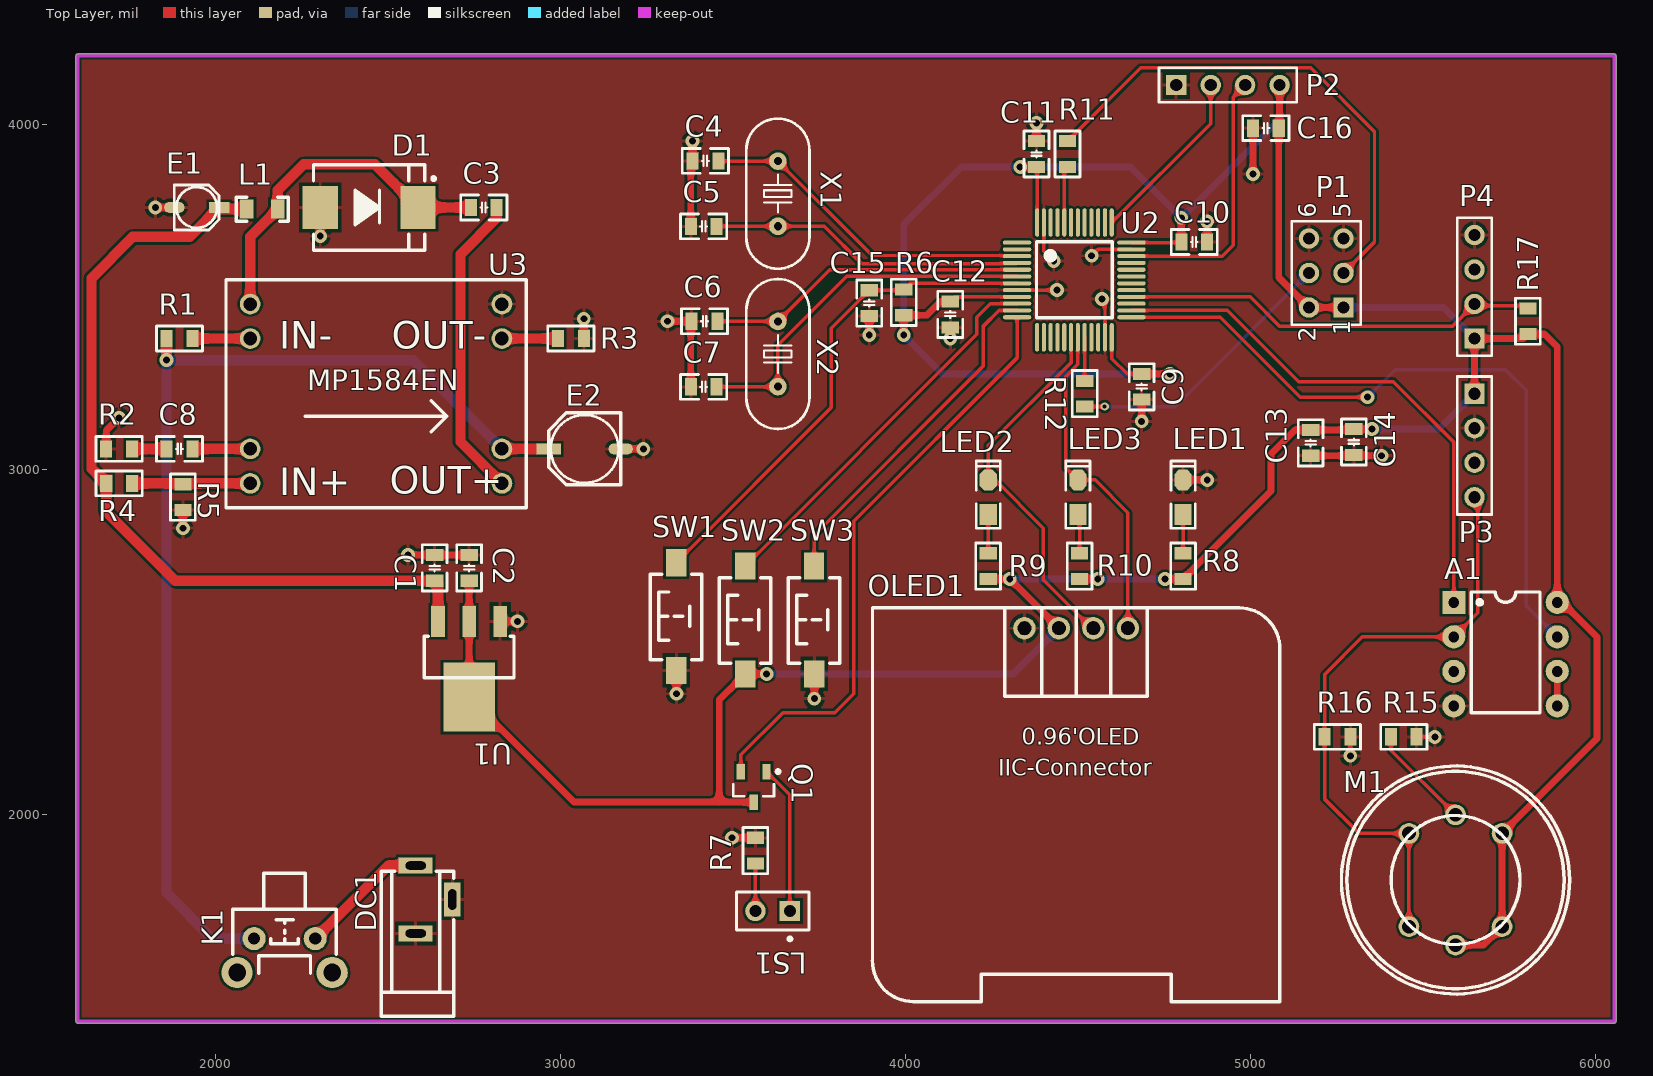
[diagram p0: Top Layer view]
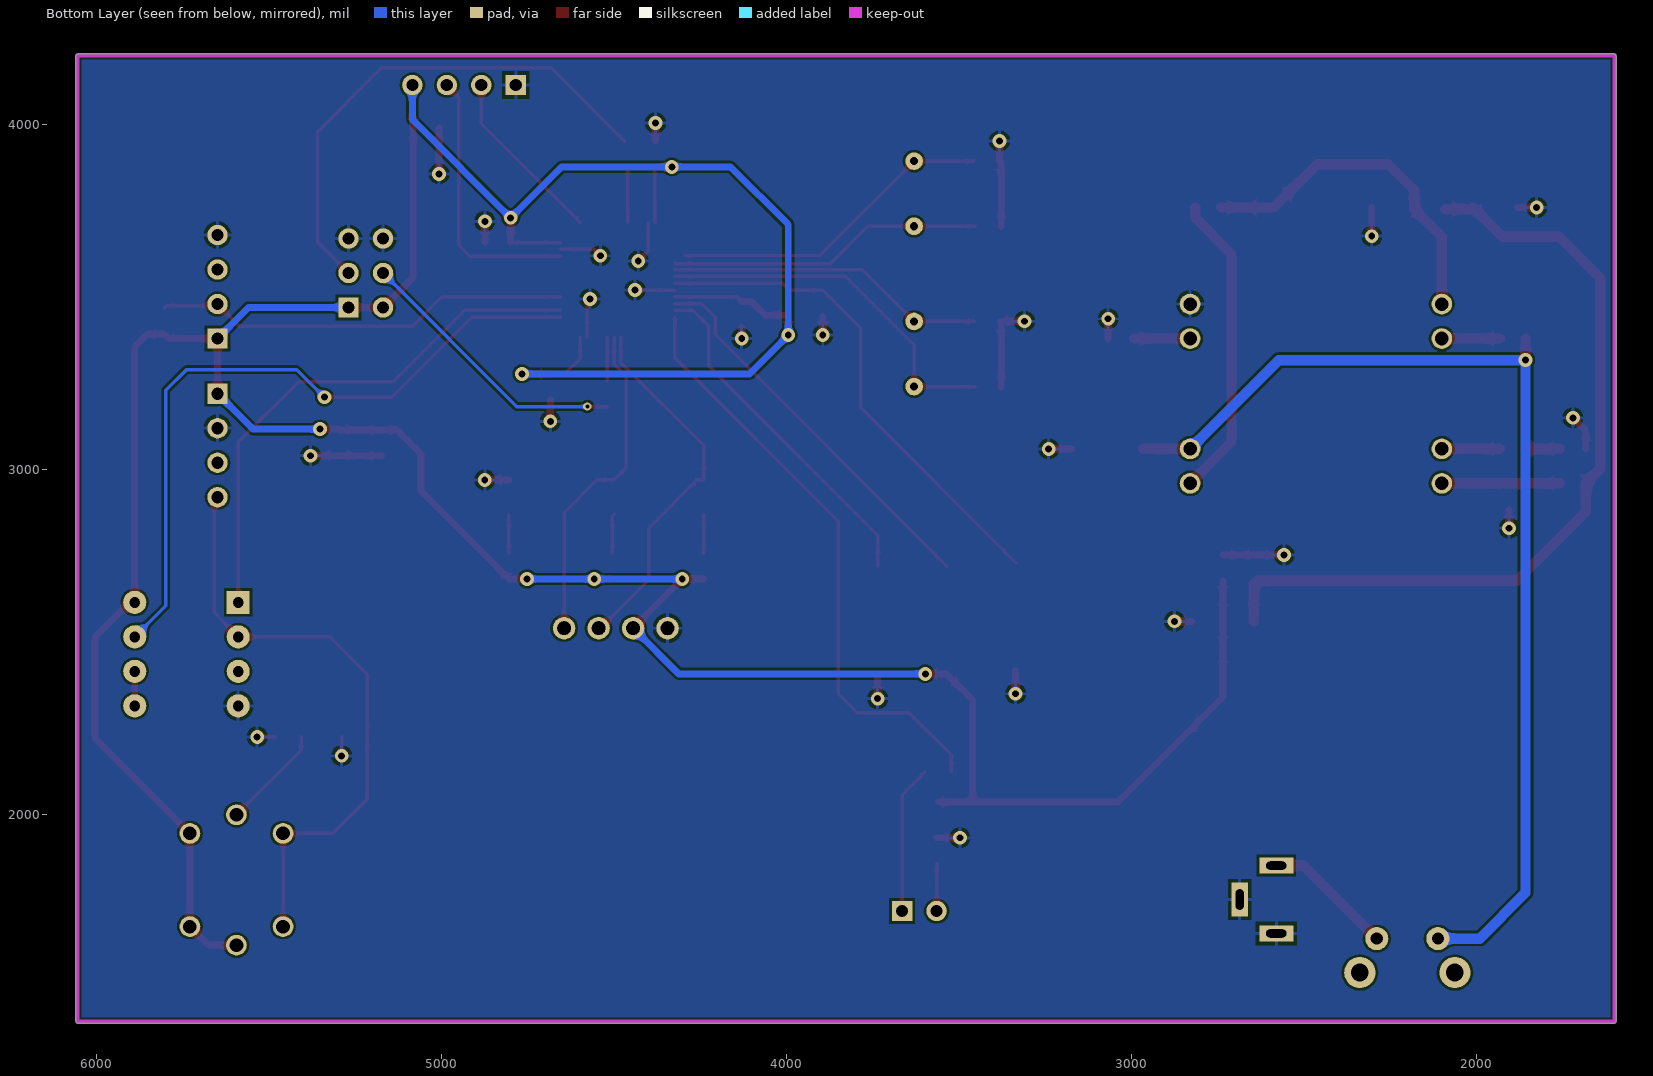
[diagram p1: Bottom Layer view, seen from below]
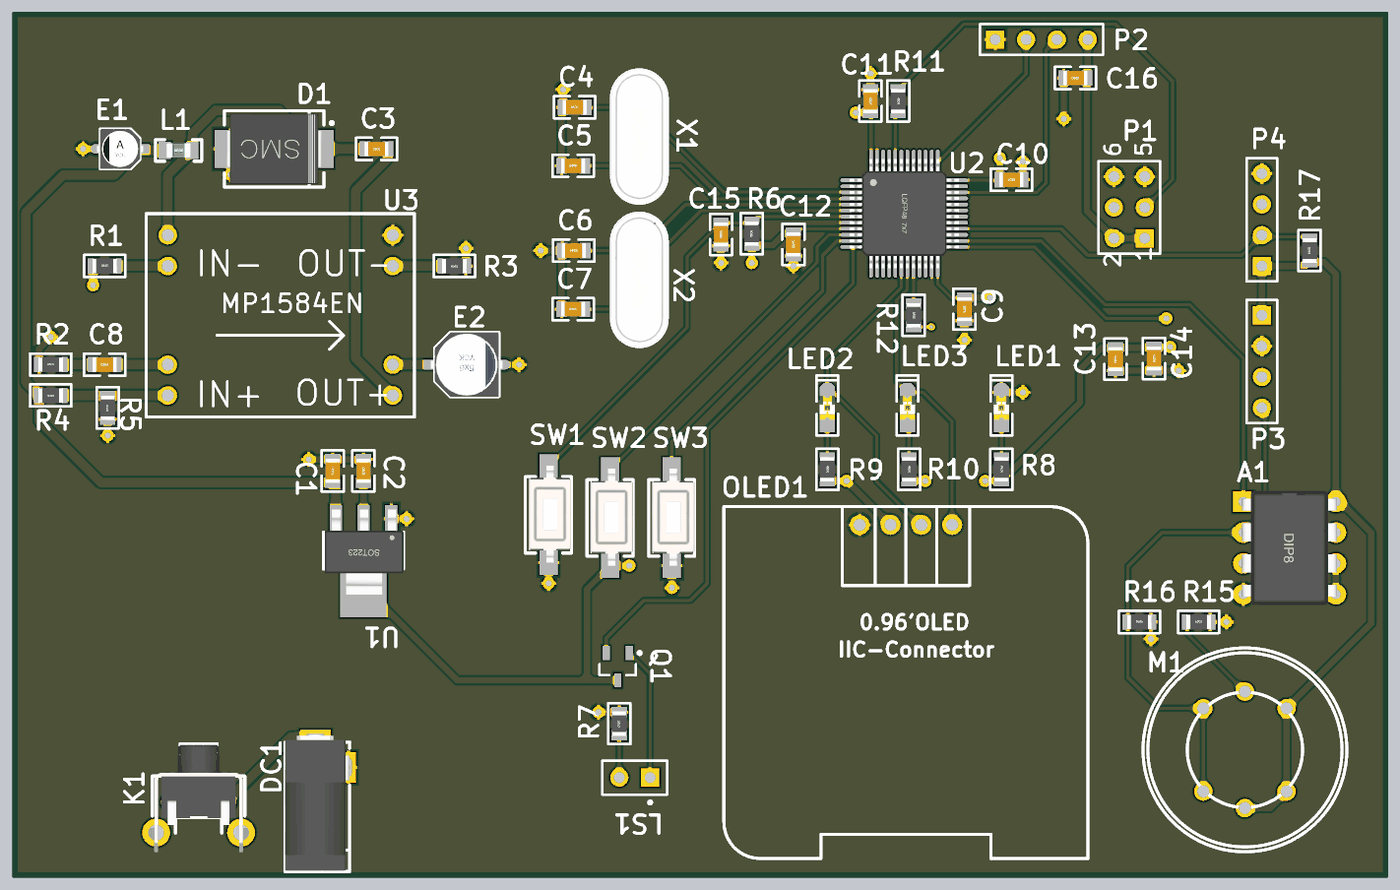
[diagram p2: 3D render of the assembled board from above, using the file's embedded part models]
# Altium PCB MISC82066.PcbDoc
Units mil, origin at the board's own origin, x right, y up, seen from the top; angles counter-clockwise.
Board outline 4465.32 x 2810.03 mil, 2 copper layers (Top Layer, Bottom Layer); 57 components, 39 nets, 194 pads, 39 vias.

## Layer stack, top to bottom (the 12.6 mil dielectric is the usual default, probably not edited)
Top Solder: solder mask 0.4, Solder Resist, Dk 3.5
Top Layer: signal copper 1.4
Dielectric 1: dielectric 12.6, FR-4, Dk 4.8
Bottom Layer: signal copper 1.4
Bottom Solder: solder mask 0.4, Solder Resist, Dk 3.5

## Board outline
1594.98,1400 ccw(c1600,1400) 1600,1394.98 6055.29,1394.98 ccw(c6055.29,1400) 6060.31,1400 6060.31,4200 ccw(c6055.29,4200) 6055.29,4205.02 1600,4205.02 ccw(c1600,4200) 1594.98,4200

## Design rules (kind name [scope] priority, off if disabled: settings)
Clearance [All] p1: gap=7
HoleSize [All] p1: absolutevalues=TRUE maxlimit=3333 minlimit=1 maxpercent=80.000 minpercent=20.000
MinimumSolderMaskSliver [All] p1: minsoldermaskwidth=0
PolygonConnect [All] p1: connectstyle=Relief reliefconductorwidth=10 reliefentries=4 polygonreliefangle="90 Angle" airgapwidth=10
RoutingVias [All] p1: holewidth=28 width=50 viastyle="Through Hole" minholewidth=28 minwidth=50 maxholewidth=28 maxwidth=50
SilkToSilkClearance [All] p1: silktosilkclearance=0
SilkToSolderMaskClearance [IsPad] p1: minsilkscreentomaskgap=0 clearancetoexposedcopper=TRUE
SolderMaskExpansion [All] p1: expansion=4
Width [All] p1: maxlimit=30 minlimit=10 preferedwidth=10
26 further rules are at their usual default settings.

## Components (designator, comment, footprint, x,y, rotation, side; value= is the part's Value field where it differs from the comment)
A1 "ADC0832" DIP8 5740,2465 r0 top
C1 "100nF" "C 0805_L" 2635,2715 r270 top
C2 "100nF" "C 0805_L" 2735,2715 r270 top
C3 "100nF" "C 0805_L" 2777.4,3760 r0 top
C4 "10PF" "C 0805_L" 3420,3895 r0 top
C5 "10PF" "C 0805_L" 3415,3705 r0 top
C6 "22PF" "C 0805_L" 3417.4,3430 r0 top
C7 "22PF" "C 0805_L" 3415,3240 r0 top
C8 "150PF" "C 0805_L" 1895,3060 r0 top
C9 "22UF" "C 0805_L" 4685,3240 r90 top
C10 "100nF" "C 0805_L" 4837.4,3660 r180 top
C11 "100nF" "C 0805_L" 4380,3915 r270 top
C12 "100nF" "C 0805_L" 4130,3450 r90 top
C13 "100nF" "C 0805_L" 5175,3077.6 r90 top
C14 "100nF" "C 0805_L" 5300,3080 r90 top
C15 "100nF" "C 0805_L" 3895,3482.6 r90 top
C16 "100nF" "C 0805_L" 5045,3990 r0 top
D1 "SS34" SMC 2445,3760 r0 top
DC1 "DC_Socket" DC-002 2580,1851.85 r270 top
E1 "22uF" "CM A(3*5.4)" 1945,3760 r0 top
E2 "220UF" "CT 5*6 - C" 3070,3060 r180 top
K1 "6x6x5" "TSW DIP-6*6*6_V" 2200,1640 r180 top
L1 "15uH" "L 0805" 2135,3755 r0 top
LED1 "Red" "LED 0805G" 4805,2920 r90 top
LED2 "Red" "LED 0805G" 4240,2920 r90 top
LED3 "Red" "LED 0805G" 4500,2920 r90 top
LS1 "Speaker" PIN2 3665,1720 r180 top
M1 "MQ-2" MQ-2 5595,1810 r0 top
OLED1 "0.96OLED_4P_MODULE_JX" 0.96OLED_4P 4495.05,2028.3 r0 top
P1 "Header 3X2" HDR2X3 5270,3470 r90 top
P2 "Header 4" HDR1X4 4785,4115 r0 top
P3 "Header 4" HDR1X4 5650,3220 r270 top
P4 "Header 4" HDR1X4 5650,3380 r90 top
Q1 "PNP" SOT-23B_N 3560,2080 r270 top
R1 "100K" "R 0805_L" 1895,3380 r0 top
R2 "100K" "R 0805_L" 1720,3060 r0 top
R3 "100K" "R 0805_L" 3030,3380 r180 top
R4 "43K" "R 0805_L" 1720,2960 r180 top
R5 "8.2K" "R 0805_L" 1905,2920 r90 top
R6 "10K" "R 0805_L" 3995,3485 r90 top
R7 "20K" "R 0805_L" 3565,1895 r90 top
R8 "300" "R 0805_L" 4805,2720 r270 top
R9 "300" "R 0805_L" 4240,2720 r270 top
R10 "300" "R 0805_L" 4505,2720 r270 top
R11 "10K" "R 0805_L" 4470,3915 r270 top
R12 "10K" "R 0805_L" 4520,3220 r270 top
R15 "4.7K" "R 0805_L" 5445,2225 r0 top
R16 "1K" "R 0805_L" 5252.6,2225 r0 top
R17 "4.7K" "R 0805_L" 5805,3430 r90 top
SW1 "3x6x5" "TSW SMD-3*6*2.5" 3335,2575 r90 top
SW2 "3x6x5" "TSW SMD-3*6*2.5" 3535,2565 r90 top
SW3 "3x6x5" "TSW SMD-3*6*2.5" 3735,2565 r90 top
U1 "AMS1117" SOT223 2735,2560 r180 top
U2 "STM32F103C8T6" "LQFP48 7X7" 4490,3550 r270 top
U3 "MP1584EN" MP1548EN 2465,3220 r0 top
X1 "32.768KHZ" "OSC HC-49S" 3630,3800 r270 top
X2 "8MHZ" "OSC HC-49S" 3630,3335 r270 top

## Footprints (in the part's own frame and the unit in brackets; to place one, negate y for a bottom-side part, rotate by r counter-clockwise, add the part's x,y. Pads: shape width x height; smd on the part's side, far side on the other; paste and mask are expansions set on the pad)
0.96OLED_4P [mm]
  round 1.65 hole 1 slot 1.005 at 0 deg paste+0 mask+0.051: 1(-3.811,12.997) 2(-1.271,13) 3(1.269,13) 4(3.809,13)
  silkscreen extent -15,-14.5 15,14.5
"C 0805_L" [mil] "无极性贴片电容"
  rect 35x50 smd: 1(-37.4,0) 2(37.4,0)
  silkscreen extent -67,-36 67,36, body extent -39,-24 39,24, height 20
"CM A(3*5.4)" [mm] "贴片电解电容，直径3mm，高5.4mm"
  rect 1.5x0.8 smd: 1(1.651,0)
  oval 1.5x0.8 smd: 2(-1.65,0)
  silkscreen extent -1.65,-1.65 1.65,1.65, body extent -1.9,-1.65 1.9,1.65, height 5.4
"CT 5*6 - C" [mm] "直径5mm，高6mm"
  rect 1.8x0.8 smd: 1(2.65,0)
  oval 1.8x0.8 smd: 2(-2.65,0)
  silkscreen extent -2.65,-2.65 2.65,2.65, body extent -2.95,-2.65 2.95,2.65, height 6
DC-002 [mm] "3.5X1.1mm"
  rect 1.2x2.5 hole 0.6 slot 1.5 at 90 deg: 1(0,0) 2(5,0)
  rect 2.5x1.2 hole 0.6 slot 1.5 at 0 deg: 3(2.5,2.7)
  silkscreen extent 0.43,-2.54 11.1,2.79, body extent -0.25,-2.55 11.05,2.8, height 7.3
DIP8 [mm]
  rect 1.7x1.7 hole 0.8: 1(-3.81,3.81)
  round 1.7 hole 0.8: 2(-3.81,1.27) 3(-3.81,-1.27) 4(-3.81,-3.81) 5(3.81,-3.81) 6(3.81,-1.27) 7(3.81,1.27) 8(3.81,3.81)
  silkscreen extent -2.54,-4.32 2.54,4.57, body extent -3.94,-4.7 3.91,4.7, height 4.5
HDR1X4 [mm] "Connector; Header; 4 Position"
  rect 1.5x1.5 hole 0.9: 1(0,0)
  round 1.5 hole 0.9: 2(2.54,0) 3(5.08,0) 4(7.62,0)
  silkscreen extent -1.27,-1.27 8.89,1.27
HDR2X3 [mm] "Connector; Header; 3x2 Position"
  rect 1.5x1.5 hole 0.9: 1(0,0)
  round 1.5 hole 0.9: 2(0,2.54) 3(2.54,0) 4(2.54,2.54) 5(5.08,0) 6(5.08,2.54)
  silkscreen extent -1.27,-1.27 6.35,3.81
"L 0805" [mil] "小功率贴片电感"
  rect 40x55 smd: 1(-45,0) 2(45,0)
  silkscreen extent -75,-35 75,35, body extent -39,-24 39,24, height 35
"LED 0805G" [mil] "绿色0805LED"
  rect 60x50 smd: 1(-50,0)
  oct 60x50 smd: 2(50,0)
  silkscreen extent -90,-35 105,35, body extent -39,-25 39,25, height 32
"LQFP48 7X7" [mm]
  oval 0.3x2.1 smd: 1(-2.75,-4.227) 2(-2.25,-4.227) 3(-1.75,-4.227) 4(-1.25,-4.227) 5(-0.75,-4.227) 6(-0.25,-4.227) 7(0.25,-4.227) 8(0.75,-4.227) 9(1.25,-4.227) 10(1.75,-4.227) 11(2.25,-4.227) 12(2.75,-4.227) 25(2.75,4.202) 26(2.25,4.202) 27(1.75,4.202) 28(1.25,4.202) 29(0.75,4.202) 30(0.25,4.202) 31(-0.25,4.202) 32(-0.75,4.202) 33(-1.25,4.202) 34(-1.75,4.202) 35(-2.25,4.202) 36(-2.75,4.202)
  oval 2.1x0.3 smd: 13(4.227,-2.75) 14(4.227,-2.25) 15(4.227,-1.75) 16(4.227,-1.25) 17(4.227,-0.75) 18(4.227,-0.25) 19(4.227,0.25) 20(4.227,0.75) 21(4.227,1.25) 22(4.227,1.75) 23(4.227,2.25) 24(4.227,2.75) 37(-4.227,2.75) 38(-4.227,2.25) 39(-4.227,1.75) 40(-4.227,1.25) 41(-4.227,0.75) 42(-4.227,0.25) 43(-4.227,-0.25) 44(-4.227,-0.75) 45(-4.227,-1.25) 46(-4.227,-1.75) 47(-4.227,-2.25) 48(-4.227,-2.75)
  silkscreen extent -2.79,-2.79 2.79,2.79, body extent -4.51,-4.5 4.5,4.5, height 1.45
MP1548EN [mil]
  round 60 hole 39.37 paste+4 mask+4: 1(-365.04,260) 2(-365.04,160) 3(-365.04,-160) 4(-365.04,-260) 5(364.96,260) 6(364.96,160) 7(364.96,-160) 8(364.96,-260)
  silkscreen extent -435,-330 435,330
MQ-2 [mil]
  round 60 hole 39.37 paste+4 mask+4: 1(0,188.98) 2(-135,135) 3(-135,-135) 4(0,-188.98) 5(135,-135) 6(135,135)
  silkscreen extent -331,-331 331,331
"OSC HC-49S" [mm]
  round 1.3 hole 0.6: 1(-2.4,0) 2(2.4,0)
  silkscreen extent -5.52,-2.32 5.52,2.33, body extent -5.52,-2.32 5.53,2.33, height 4.13
PIN2 [mm] "Photosensitive Diode; 2 Leads"
  rect 1.5x1.5 hole 0.9: 1(0,0)
  round 1.5 hole 0.9: 2(2.54,0)
  silkscreen extent -1.4,-1.4 3.94,2.17
"R 0805_L" [mil] "1/8W贴片电阻"
  rect 35x50 smd: 1(-37.4,0) 2(37.4,0)
  silkscreen extent -67,-36 67,36, body extent -39,-25 39,25, height 20
SMC [mm] "7.1x5.9*2.3mm（长宽高，不包括引脚）"
  rect 2.6x3.15 smd: 1(-3.6,0) 2(3.6,0)
  silkscreen extent -4.1,-3.15 4.88,3.15, body extent -3.95,-2.9 3.95,2.9, height 2.45
SOT223 [mil]
  rect 40x90 smd: 1(-90,0) 2(0,0) 3(90,0)
  rect 150x200 smd: 2(0,220)
  silkscreen extent -130,43 130,163, body extent -130,-30 126,246, height 65
SOT-23B_N [mm] "SOT23, 3-Leads, Body 2.9x1.3mm, Pitch 0.95mm, Lead Span 2.4mm, IPC Medium Density"
  rect 1.15x0.6 smd: 1(-1.125,0.95) 2(-1.125,-0.95) 3(1.125,0)
  silkscreen extent -1.25,-1.5 0.7,1.93, body extent -0.7,-1.5 0.7,1.5, height 1.14
"TSW DIP-6*6*6_V" [mm] "侧按轻触开关 6*6*6mm"
  round 2.3 hole 1.3: 0(-3.5,2.5) 0(3.5,2.5)
  round 1.7 hole 0.9: 1(-2.25,0) 2(2.25,0)
  silkscreen extent -3.81,-4.83 3.81,2.54, body extent -4.18,-4.72 4.18,4.13, height 7.47
"TSW SMD-3*6*2.5" [mm] "3*6*2.5mm"
  rect 2x1.5 smd: 1(-3.996,-0.02) 2(3.937,0)
  silkscreen extent -3.21,-1.9 3.09,1.9, body extent -4,-1.88 4,1.62, height 2.59

## Part data
C1 C2 C3 C4 C5 C6 C7 C8 C9 C10 C11 C12 C13 C14 C15 C16: library part C, "SMD capacitor"
D1: "Schottky diode"
E1: library part CE_SMD, "SMD electrolytic capacitor"
E2: library part CS_SMD, "SMD solid-state capacitor"
K1: library part "TSW DIP-6x6_V", "Side-push through-hole 6x6 tact switch"
L1: library part L, "Low-power SMD inductor"
LED1 LED2 LED3: library part LED-SMD, "SMD LED"
LS1: "Loudspeaker"
M1: "Gas sensor"
P1: "Header, 3-Pin, Dual row"
P2 P3 P4: "Header, 4-Pin"
Q1: "PNP Bipolar Transistor"
R1 R2 R3 R4 R5 R6 R7 R8 R9 R10 R11 R12 R15 R16 R17: library part R, "SMD resistor"
SW1 SW2 SW3: library part "TSW 3x6", "3x6 tact switch"
U1: "Three-terminal regulator IC"
X1 X2: library part XTAL-2P, "2-pin passive crystal oscillator"

## Via types
v1: diameter 40, hole 20, Top Layer to Bottom Layer, 38 vias
v2: diameter 24, hole 12, Top Layer to Bottom Layer, 1 vias

## Nets (pads, with @x,y where several pads share a name; then routed paths per layer and width w, separated by ;. In a path a pad name is that pad's centre, name@x,y a point inside that pad or via, vN(x,y) a via of type N, cw(c..) or ccw(c..) an arc to the next point about the centre after c; other vN are vias at no path point)
3V3: A1.8 C2.2 C9.2 C10.2 C11.2 C12.2 C13.2 C14.2 C16.2 M1.4 M1.5 M1.6 OLED1.2 P1.1 P1.2 P2.4 P3.1 P4.1 Q1.3 R6.1 R8.2 R9.2 R10.2 R17.1 SW2.1 U1.2 U2.9 U2.24 U2.36 U2.48 | length 11893.6
  Top Layer w10: C12.2 4143.39,3500.79 U2.9 ; C11.2 4381.73,3875.87 U2.48 ; U2.24 4598.27,3321.73 4642.6,3277.4 C9.2 ; U2.36 4798.27,3658.27 C10.2
  Top Layer w20: C2.2 2735,2340 3039.29,2035.71 3460,2035.71 ; Q1.3 3460,2035.71 ; v1(3597.69,2407.69) SW2.1 3460,2331.9 3460,2035.71 ; v1(3995,3390) R6.1 4062.6,3447.6 4102.4,3487.4 C12.2 ; R9.2 v1(4302.5,2682.6) OLED1.2 ; v1(4332.6,3877.6) C11.2 ; R10.2 v1(4557.6,2682.6) ; C9.2 v1(4767.4,3277.4) ; v1(4752.4,2682.6) R8.2 5060,2937.6 5060,3045 5130,3115 C13.2 5297.6,3115 C14.2 v1(5352.4,3117.4) ; C10.2 v1(4800,3730) ; P2.4 5085,3992.6 C16.2 5082.4,3557.6 P1.2 P1.1 ; M1.4 5676.02,1621.02 M1.5 M1.6 6005,2220 6005,2515 5905,2615 A1.8 5890,3355 5852.4,3392.6 R17.1 5792.41,3380 P4.1 P3.1
  Bottom Layer w20: v1(3597.69,2407.69) 4312.59,2407.69 OLED1.2 ; v1(4302.5,2682.6) v1(4557.6,2682.6) v1(4752.4,2682.6) ; v1(4767.4,3277.4) 4107.61,3277.4 v1(3995,3390) 3995,3710 4162.6,3877.6 v1(4332.6,3877.6) 4652.4,3877.6 v1(4800,3730) 5085,4015 P2.4 ; P1.1 5560,3470 P4.1 ; v1(5352.4,3117.4) 5547.4,3117.4 P3.1
5V: C1.2 E1.1 L1.1 R4.2 U1.3 | length 2389.1
  Top Layer w30: L1.1 2015,3755 E1.1 1925,3675 1760,3675 1640,3555 1640,3002.6 R4.2 1682.6,2877.4 1882.4,2677.6 C1.2 2645,2667.6 U1.3
BOOT0: R11.2 U2.44 | length 165.1
  Top Layer w10: U2.44 4460.47,3868.08 R11.2
BOOT1: R12.1 U2.20 | length 126.4
  Top Layer w10: U2.20 4519.53,3257.87 R12.1
GND: A1.4 C1.1 C2.1 C4.1 C5.1 C6.1 C7.1 C9.1 C10.1 C11.1 C12.1 C13.1 C14.1 C15.1 C16.1 D1.1 DC1.2 DC1.3 E1.2 E2.2 LED1.2 OLED1.1 P1.5 P1.6 P2.1 P3.2 P4.4 R2.1 R3.1 R5.1 R7.2 R15.2 R16.2 SW1.1 SW3.1 U1.1 U2.8 U2.23 U2.35 U2.47 U3.5 | length 2639.6
  Top Layer w10: U2.8 v1(4439.53,3520.47) ; U2.47 4401.42,3633.58 v1(4430,3605) ; v1(4540,3620) 4558.58,3638.58 U2.35 ; v1(4570,3495) 4578.58,3486.42 U2.23 ; v1(5290,2170) R16.2 ; R15.2 v1(5535,2225)
  Top Layer w20: R2.1 1682.6,3112.6 v1(1720,3150) ; v1(1825,3760) E1.2 ; v1(1905,2830) R5.1 ; v1(2303.27,3676.73) D1.1 ; v1(2557.4,2752.4) C1.1 C2.1 ; U1.1 v1(2875,2560) ; R3.1 v1(3067.4,3437.4) ; E2.2 v1(3240,3060) ; v1(3310,3430) C6.1 3377.6,3427.6 C7.1 ; v1@3335.79,2340.79 SW1.1 ; C5.1 3377.6,3890 C4.1 v1(3382.6,3952.6) ; v1(3497.4,1932.4) R7.2 ; v1(3735.79,2335.79) SW3.1 ; v1(3895,3390) C15.1 ; v1(4130,3380) C12.1 ; C11.1 v1@4380,4015 ; v1(4685,3140) C9.1 ; LED1.2 v1(4875,2970) ; C10.1 v1(4874.8,3719.8) ; v1(5007.6,3857.4) C16.1 ; C13.1 v1(5380.2,3040.2)
  other v1: 3335.79,2350 4380,4005
NetA1_2: A1.2 M1.2 M1.3 P3.4 R16.1 | length 1775
  Top Layer w10: M1.3 M1.2 5315,1945 5215.2,2044.8 R16.1 5215.2,2405.2 5325,2515 A1.2 5660,2585 5660,2910 P3.4
NetC3_1: C3.1 D1.2 L1.2 U3.1 | length 1006
  Top Layer w30: U3.1 2099.96,3674.96 L1.2 2180,3810 2255,3885 2461.73,3885 D1.2 C3.1
NetC3_2: C3.2 U3.8 | length 893.1
  Top Layer w30: C3.2 2814.8,3729.8 2710,3625 2710,3079.96 U3.8
NetC8_1: C8.1 R2.2 | length 100.2
  Top Layer w30: R2.2 C8.1
NetC8_2: C8.2 U3.3 | length 167.6
  Top Layer w30: C8.2 U3.3
NetDC1_1: DC1.1 K1.1 | length 379.2
  Top Layer w30: K1.1 2500.43,1851.85 DC1.1
NetLED1_1: LED1.1 R8.1 | length 112.6
  Top Layer w10: R8.1 LED1.1
NetLED2_1: LED2.1 R9.1 | length 112.6
  Top Layer w10: R9.1 LED2.1
NetLED3_1: LED3.1 R10.1 | length 114.7
  Top Layer w10: LED3.1 4505,2865 R10.1
NetLS1_1: LS1.1 Q1.1 | length 432.3
  Top Layer w10: Q1.1 3665,2056.69 LS1.1
NetLS1_2: LS1.2 R7.1 | length 137.6
  Top Layer w10: LS1.2 R7.1
NetM1_1: M1.1 R15.1 | length 303.6
  Top Layer w10: R15.1 5407.6,2186.38 M1.1
NetP1_3: P1.3 R11.1 | length 1502
  Top Layer w10: R11.1 4682.59,4165 5175,4165 5360,3980 5360,3660 P1.3
NetP1_4: P1.4 R12.2 | length 810.5
  Top Layer w10: R12.2 v2(4577.6,3182.6)
  Bottom Layer w10: v2(4577.6,3182.6) 4782.6,3182.6 P1.4
NetR1_2: R1.2 U3.2 | length 167.6
  Top Layer w30: R1.2 U3.2
NetR3_2: R3.2 U3.6 | length 162.6
  Top Layer w30: U3.6 R3.2
NetR4_1: R4.1 R5.2 U3.4 | length 342.6
  Top Layer w30: R4.1 U3.4
OSC32_IN: C4.2 U2.3 X1.1 | length 951.2
  Top Layer w10: C4.2 3457.91,3894.49 X1.1 3903.81,3620.68 U2.3@4295,3620.68
OSC32_OUT: C5.2 U2.4 X1.2 | length 916.9
  Top Layer w10: C5.2 3452.91,3705.51 X1.2 3764.49,3705.51 3872.57,3597.43 4321.8,3597.43 U2.4
OSC_IN: C6.2 U2.5 X2.1 | length 931.1
  Top Layer w10: C6.2 3629.49,3430 X2.1 3780.04,3579.53 U2.5
OSC_OUT: C7.2 U2.6 X2.2 | length 1073.8
  Top Layer w10: C7.2 3629.49,3240 X2.2 3630,3360 3830,3560 4323.43,3560 U2.6
PA0: SW2.2 U2.10 | length 1133.1
  Top Layer w10: SW2.2 4207,3392 4207,3442 4246.1,3481.1 U2.10
PA1: SW3.2 U2.11 | length 1015.8
  Top Layer w10: SW3.2 3735,2810 4225,3300 4225,3415 4271.42,3461.42 U2.11
PA2: Q1.2 U2.12 | length 1737.1
  Top Layer w10: Q1.2 3522.6,2172.6 3645,2295 3795,2295 3850,2350 3850,2850 4323.58,3323.58 U2.12
PB0: LED2.2 OLED1.3 U2.18 | length 1084
  Top Layer w10: U2.18 4480.16,3310.16 4240,3070 LED2.2 4260,2970 4400,2830 4400,2680 4539.9,2540.1 OLED1.3
PB1: LED3.2 OLED1.4 U2.19 | length 961.8
  Top Layer w10: U2.19 4499.84,3304.84 4465,3270 4465,3005 LED3.2 4550,2970 4645,2875 OLED1.4
PB12: A1.7 U2.25 | length 2030.8
  Top Layer w10: U2.25 4913.27,3441.73 5145,3210 v1@5320,3210
  Bottom Layer w10: v1(5340,3210) 5420,3290 5740,3290 5800,3230 5800,2605 A1.7
PB13: A1.1 U2.26 | length 1557.6
  Top Layer w10: U2.26 4933.58,3461.42 5140,3255 5415,3255 5590,3080 A1.1
PB14: A1.5 A1.6 | length 100
  Top Layer w20: A1.5 A1.6
PB15: P4.2 R17.2 U2.28 | length 1217.3
  Top Layer w10: U2.28 4999.21,3500.79 5085,3415 5585,3415 P4.2 5655,3475 5797.4,3475 R17.2
RST: C15.2 R6.2 SW1.2 U2.7 | length 1458.9
  Top Layer w10: SW1.2 3785,3180 3785,3410 C15.2 3992.6,3520 R6.2 4012.76,3540.16 U2.7
SWCLK: P2.2 U2.37 | length 517.4
  Top Layer w10: U2.37 4885,4003.15 P2.2
SWDIO: P2.3 U2.34 | length 787
  Top Layer w10: U2.34 4918.9,3618.9 4950,3650 4950,4080 P2.3
VIN: E2.1 K1.2 R1.1 U3.7 | length 3131
  Top Layer w30: v1(1857.6,3317.4) R1.1 ; U3.7 E2.1
  Bottom Layer w30: K1.2 1990,1640 1857.6,1772.4 v1(1857.6,3317.4) 2572.56,3317.4 U3.7
pads on no net: A1.3 K1.0 P3.3 P4.3 U2.1 U2.2 U2.13 U2.14 U2.15 U2.16 U2.17 U2.21 U2.22 U2.27 U2.29 U2.30 U2.31 U2.32 U2.33 U2.38 U2.39 U2.40 U2.41 U2.42 U2.43 U2.45 U2.46

## Polygon pours and split planes (outlines as drawn)
GND on Bottom Layer "G" (solid, remove dead copper, pour order 6): 1535,4260 6090,4260 6180,4350 6230,4300 6230,1090 1605,1090 1470,1225
GND on Top Layer "G" (solid, remove dead copper, pour order 8): 1355,4375 1425,4305 6210,4305 6210,1280 6175,1245 6160,1230 1340,1230

## Keep-outs
Keep-Out Layer:
  lines w10: 1600,3155 1600,2975 ; 5100,4200 6055.29,4200 6055.29,1400 1600,1400 1600,2975 ; 5200,4200 1600,4200 1600,2975